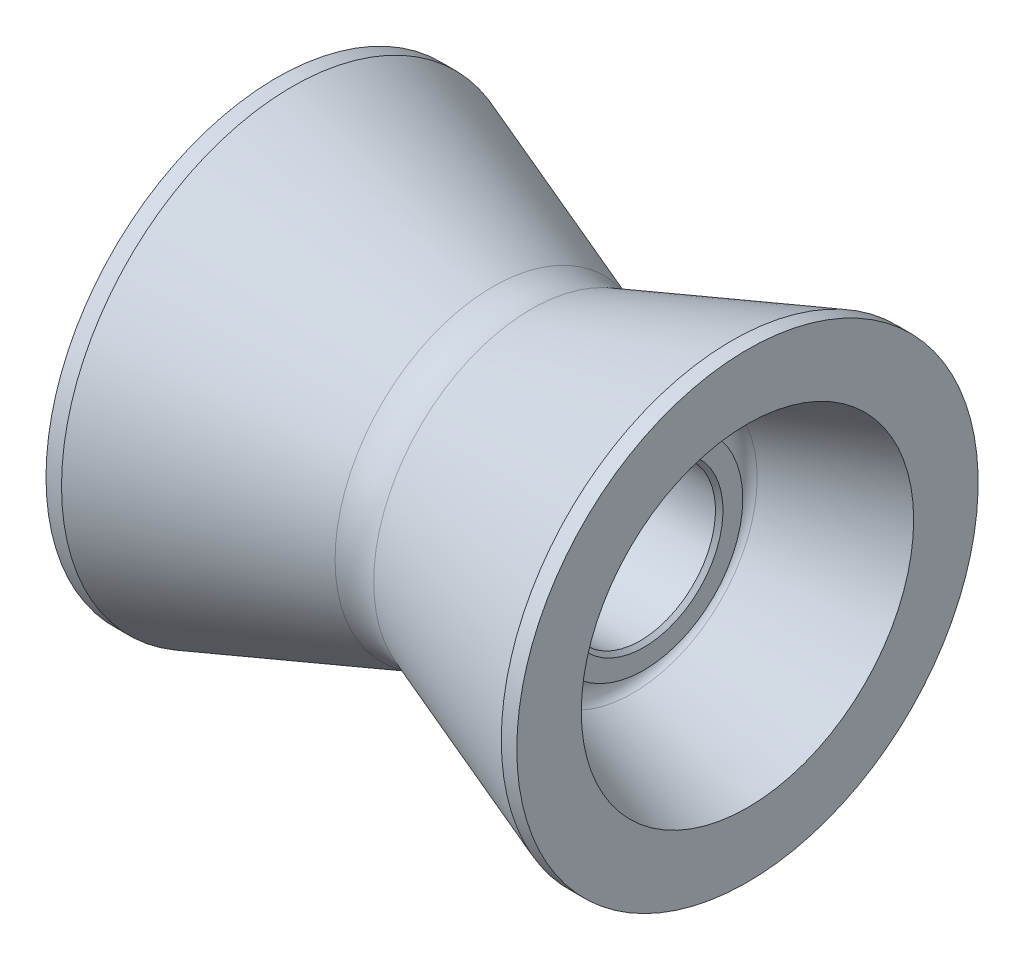
SolidWorks part; units mm, degrees
ref_plane "Front Plane" through (0, 0, 0) normal (0, 0, 1) x (1, 0, 0)
ref_plane "Top Plane" through (0, 0, 0) normal (0, 1, 0) x (1, 0, 0)
ref_plane "Right Plane" through (0, 0, 0) normal (1, 0, 0) x (0, 0, -1)
sketch "Sketch1" plane through (0, 0, 0) normal (0, 0, 1) x (1, 0, 0)
  line L0 (-142.4333, 0) -> (142.4333, 0) construction
  line L1 (0, 0) -> (0, 127.1282) construction
  line L2 (-125, 122.5) -> (-116.7678, 122.5)
  line L3 (-116.7678, 122.5) -> (-10.2606, 83.7346)
  line L4 (-125, 122.5) -> (-125, 88.2501)
  line L5 (-125, 88.2501) -> (-64.0824, 66.0778)
  line L6 (-70, 52.5) -> (-70, 0)
  line L7 (-70, 52.5) -> (-66.4765, 52.5)
  line L8 (70, 52.5) -> (66.4765, 52.5)
  line L9 (70, 52.5) -> (70, 0)
  line L10 (125, 88.2501) -> (64.0824, 66.0778)
  line L11 (125, 122.5) -> (125, 88.2501)
  line L12 (116.7678, 122.5) -> (10.2606, 83.7346)
  line L13 (125, 122.5) -> (116.7678, 122.5)
  line L14 (-70, 0) -> (70, 0)
  arc A0 (-66.4765, 52.5) -> (-64.0824, 66.0778) centre (-66.4765, 59.5) ccw
  arc A1 (66.4765, 52.5) -> (64.0824, 66.0778) centre (66.4765, 59.5) cw
  arc A2 (10.2606, 83.7346) -> (-10.2606, 83.7346) centre (0, 111.9253) cw
  point P4 (0, 0)
  point P36 (-125, 105.375)
  point P40 (0, 80)
  dimension "D1" = 14
  dimension "D9" = 30
  dimension "D2" = 52.5
  dimension "D3" = 35
  dimension "D4" = 80
  dimension "D5" = 250
  dimension "D6" = 55
  dimension "D7" = 122.5
  dimension "D8" = 140
revolve "Revolve1" add sketch "Sketch1" angle 360 about L14
sketch "Sketch2" plane through (-70, 0, 0) normal (-1, 0, 0) x (0, 0, 1)
  line L0 (0, 0) -> (0, 104.7492) construction
  line L1 (-11, 45.4) -> (11, 45.4)
  line L2 (-11, 45.4) -> (-11, 38.4578)
  line L3 (11, 45.4) -> (11, 38.4578)
  arc A0 (-11, 38.4578) -> (11, 38.4578) centre (0, 0) ccw
  point P7 (0, 45.4)
  dimension "D1" = 80
  dimension "D2" = 45.4
  dimension "D3" = 22
extrude "Cut-Extrude1" cut sketch "Sketch2" against normal through all
chamfer "Chamfer1" distance 2 angle 45 2 edges at (70, -40, 0) (-70, -40, 0)
fillet "Fillet1" radius 0.5 2 edges at (0, 45.4, 11) (0, 45.4, -11)
